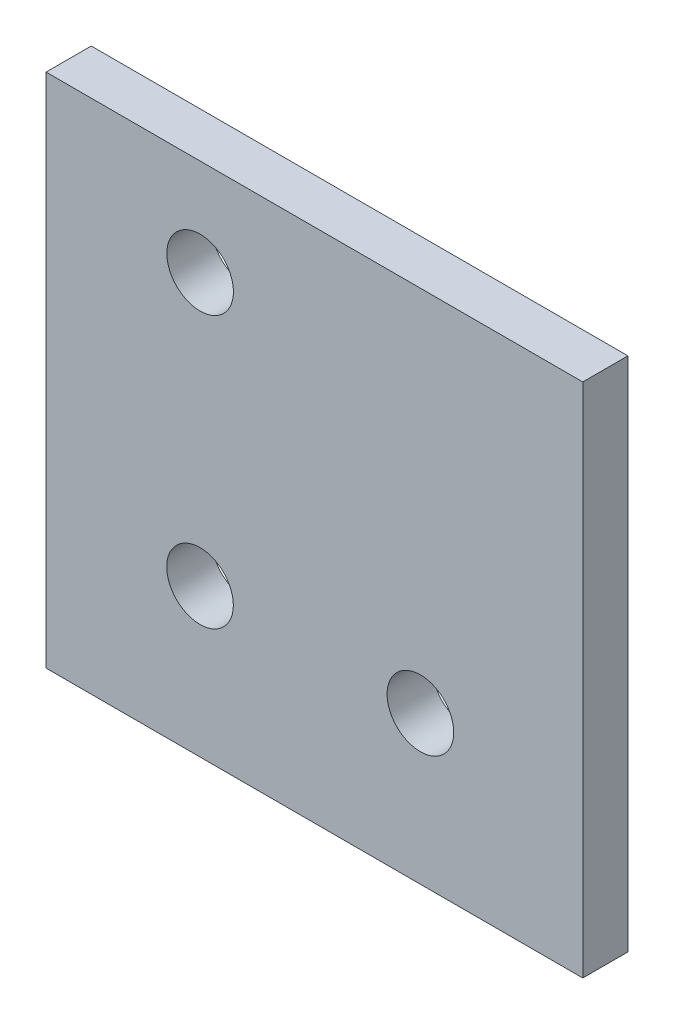
from build123d import *

# Parameters (mm, degrees)
SKETCH1_W           = 166.35
SKETCH1_H           = 160
SKETCH1_R           = 10.325
BOSS_EXTRUDE1_DEPTH = 14


with BuildPart() as part:
    # Sketch1 → Boss-Extrude1 (new body)
    with BuildSketch(Plane.XY):
        Rectangle(SKETCH1_W, SKETCH1_H)
        with Locations((-35.423, 50.048)):
            Circle(SKETCH1_R, mode=Mode.SUBTRACT)
        with Locations((-35.455423125, -34.102)):
            Circle(SKETCH1_R, mode=Mode.SUBTRACT)
        with Locations((32.852, -34.102)):
            Circle(SKETCH1_R, mode=Mode.SUBTRACT)
    extrude(amount=BOSS_EXTRUDE1_DEPTH)


solid = part.part
